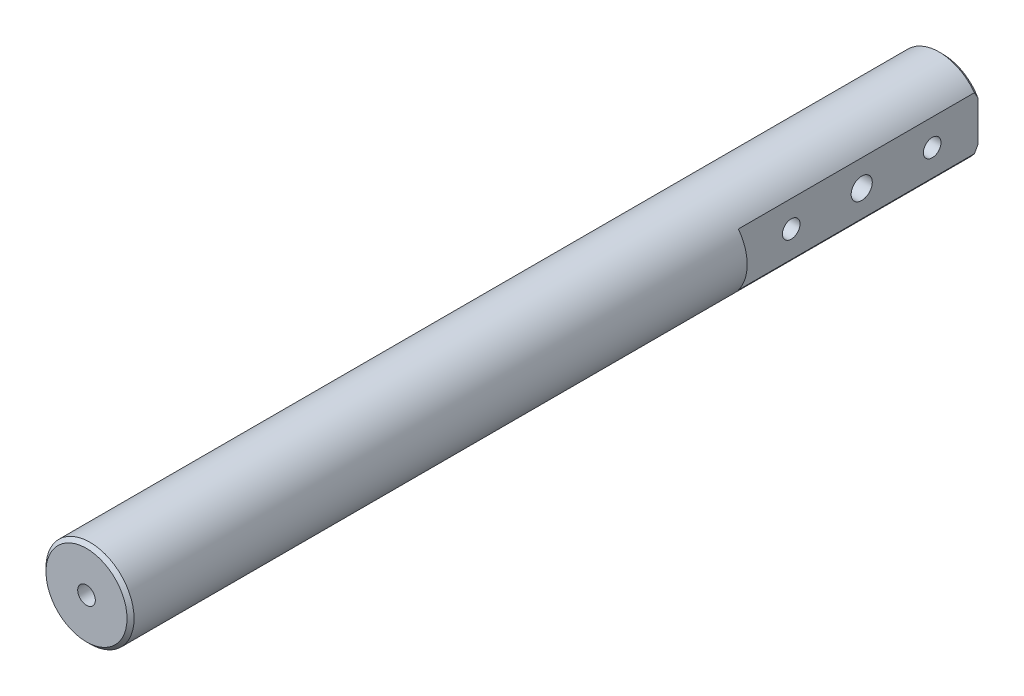
SolidWorks part; units mm, degrees
material "硬质光圆"
ref_plane "Front Plane" through (0, 0, 0) normal (0, 0, 1) x (1, 0, 0)
ref_plane "Top Plane" through (0, 0, 0) normal (0, 1, 0) x (1, 0, 0)
ref_plane "Right Plane" through (0, 0, 0) normal (1, 0, 0) x (0, 0, -1)
sketch "Sketch1" plane through (0, 0, 0) normal (0, 0, 1) x (1, 0, 0)
  circle A0 centre (0, 0) radius 12.5
  dimension "D1" = 25
extrude "Boss-Extrude1" add sketch "Sketch1" along normal blind 243
sketch "Sketch2" plane through (0, 0, 0) normal (0, 0, 1) x (1, 0, 0)
  line L1 (10, 7.5) -> (30, 7.5)
  line L2 (10, 7.5) -> (10, -7.5)
  line L3 (10, -7.5) -> (30, -7.5)
  line L4 (30, 7.5) -> (30, -7.5)
  circle A0 centre (0, 0) radius 12.5 construction
  dimension "D1" = 10
  dimension "D2" = 20
extrude "Cut-Extrude1" cut sketch "Sketch2" along normal blind 68
hole_wizard "M6 Tapped Hole1" positions "Sketch4" profile "Sketch3" tap size "M6" standard "Gb"
sketch "Sketch4" plane through (0, 0, 243) normal (0, 0, 1) x (1, 0, 0)
  point P0 (0, 0)
sketch "Sketch3" plane through (0, 0, 243) normal (1, 0, 0) x (0, -1, 0)
  line L0 (0, 0) -> (0, 16.5022)
  line L1 (0, 16.5022) -> (2.5, 15)
  line L2 (2.5, 15) -> (2.5, 0)
  line L5 (2.5, 0) -> (0, 0)
  line L10 (0, 16.5022) -> (-2.5, 15) construction
  line L11 (0, -6.35) -> (0, 107.95) construction
  dimension "螺纹孔钻头直径" = 5
  dimension "螺纹孔钻头深度" = 15
  dimension "导头角度" = 118
cosmetic thread "Hole thread 1" parameters "D1"=12, "D2"=6
hole_wizard "M6 Tapped Hole2" positions "Sketch6" profile "Sketch5" tap size "M6" standard "Gb"
sketch "Sketch6" plane through (10, 0, 0) normal (1, 0, 0) x (0, 0, -1)
  line L0 (-68, 0) -> (0, 0) construction
  line L1 (-68, 7.5) -> (-68, -7.5) construction
  line L2 (0, 7.5) -> (0, -7.5) construction
  point P0 (-13, 0)
  point P2 (-53, 0)
  dimension "D1" = 13
  dimension "D2" = 40
sketch "Sketch5" plane through (10, 0, 13) normal (0, 1, 0) x (0, 0, -1)
  line L0 (0, 0) -> (0, 16.5022)
  line L1 (0, 16.5022) -> (2.5, 15)
  line L2 (2.5, 15) -> (2.5, 0)
  line L5 (2.5, 0) -> (0, 0)
  line L10 (0, 16.5022) -> (-2.5, 15) construction
  line L11 (0, -6.35) -> (0, 107.95) construction
  dimension "螺纹孔钻头直径" = 5
  dimension "螺纹孔钻头深度" = 15
  dimension "导头角度" = 118
cosmetic thread "Hole thread 2" parameters "D1"=12, "D2"=6
cosmetic thread "Hole thread 3" parameters "D1"=12, "D2"=6
sketch "Sketch7" plane through (0, 0, 0) normal (0, 0, -1) x (-1, 0, 0)
  line L1 (10, -7.5) -> (12.5, -7.5)
  line L2 (10, -7.5) -> (10, 7.5)
  line L3 (10, 7.5) -> (12.5, 7.5)
  line L4 (12.5, -7.5) -> (12.5, 7.5)
  arc A0 (-10, -7.5) -> (-10, 7.5) centre (0, 0) ccw construction
  dimension "D1" = 10
extrude "Cut-Extrude2" cut sketch "Sketch7" against normal blind 160
hole_wizard "M4 Tapped Hole1" positions "Sketch9" profile "Sketch8" tap size "M4" standard "Gb"
sketch "Sketch9" plane through (-10, 0, 0) normal (-1, 0, 0) x (0, 0, 1)
  line L0 (0, 0) -> (150.7352, 0) construction
  line L1 (0, 7.5) -> (0, -7.5) construction
  point P0 (8, 0)
  point P2 (83, 0)
  point P13 (48, 0)
  dimension "D1" = 8
  dimension "D2" = 75
  dimension "D3" = 40
sketch "Sketch8" plane through (-10, 0, 8) normal (0, 1, 0) x (0, 0, 1)
  line L0 (0, 0) -> (0, 11.0914)
  line L1 (0, 11.0914) -> (1.65, 10.1)
  line L2 (1.65, 10.1) -> (1.65, 0)
  line L5 (1.65, 0) -> (0, 0)
  line L10 (0, 11.0914) -> (-1.65, 10.1) construction
  line L11 (0, -6.35) -> (0, 107.95) construction
  dimension "螺纹孔钻头直径" = 3.3
  dimension "螺纹孔钻头深度" = 10.1
  dimension "导头角度" = 118
cosmetic thread "Hole thread 4" parameters "D1"=8, "D2"=4
cosmetic thread "Hole thread 5" parameters "D1"=8, "D2"=4
cosmetic thread "Hole thread 7" parameters "D1"=8, "D2"=4
sketch "Sketch10" plane through (10, 0, 0) normal (1, 0, 0) x (0, 0, -1)
  line L0 (-53, 0) -> (-13, 0) construction
  circle A0 centre (-33, 0) radius 3
  dimension "D1" = 6
extrude "Cut-Extrude3" cut sketch "Sketch10" against normal blind 10
chamfer "Chamfer1" distance 1 angle 45 3 edges at (0, 12.5, 0) (0, -12.5, 0) (12.5, 0, 243)
